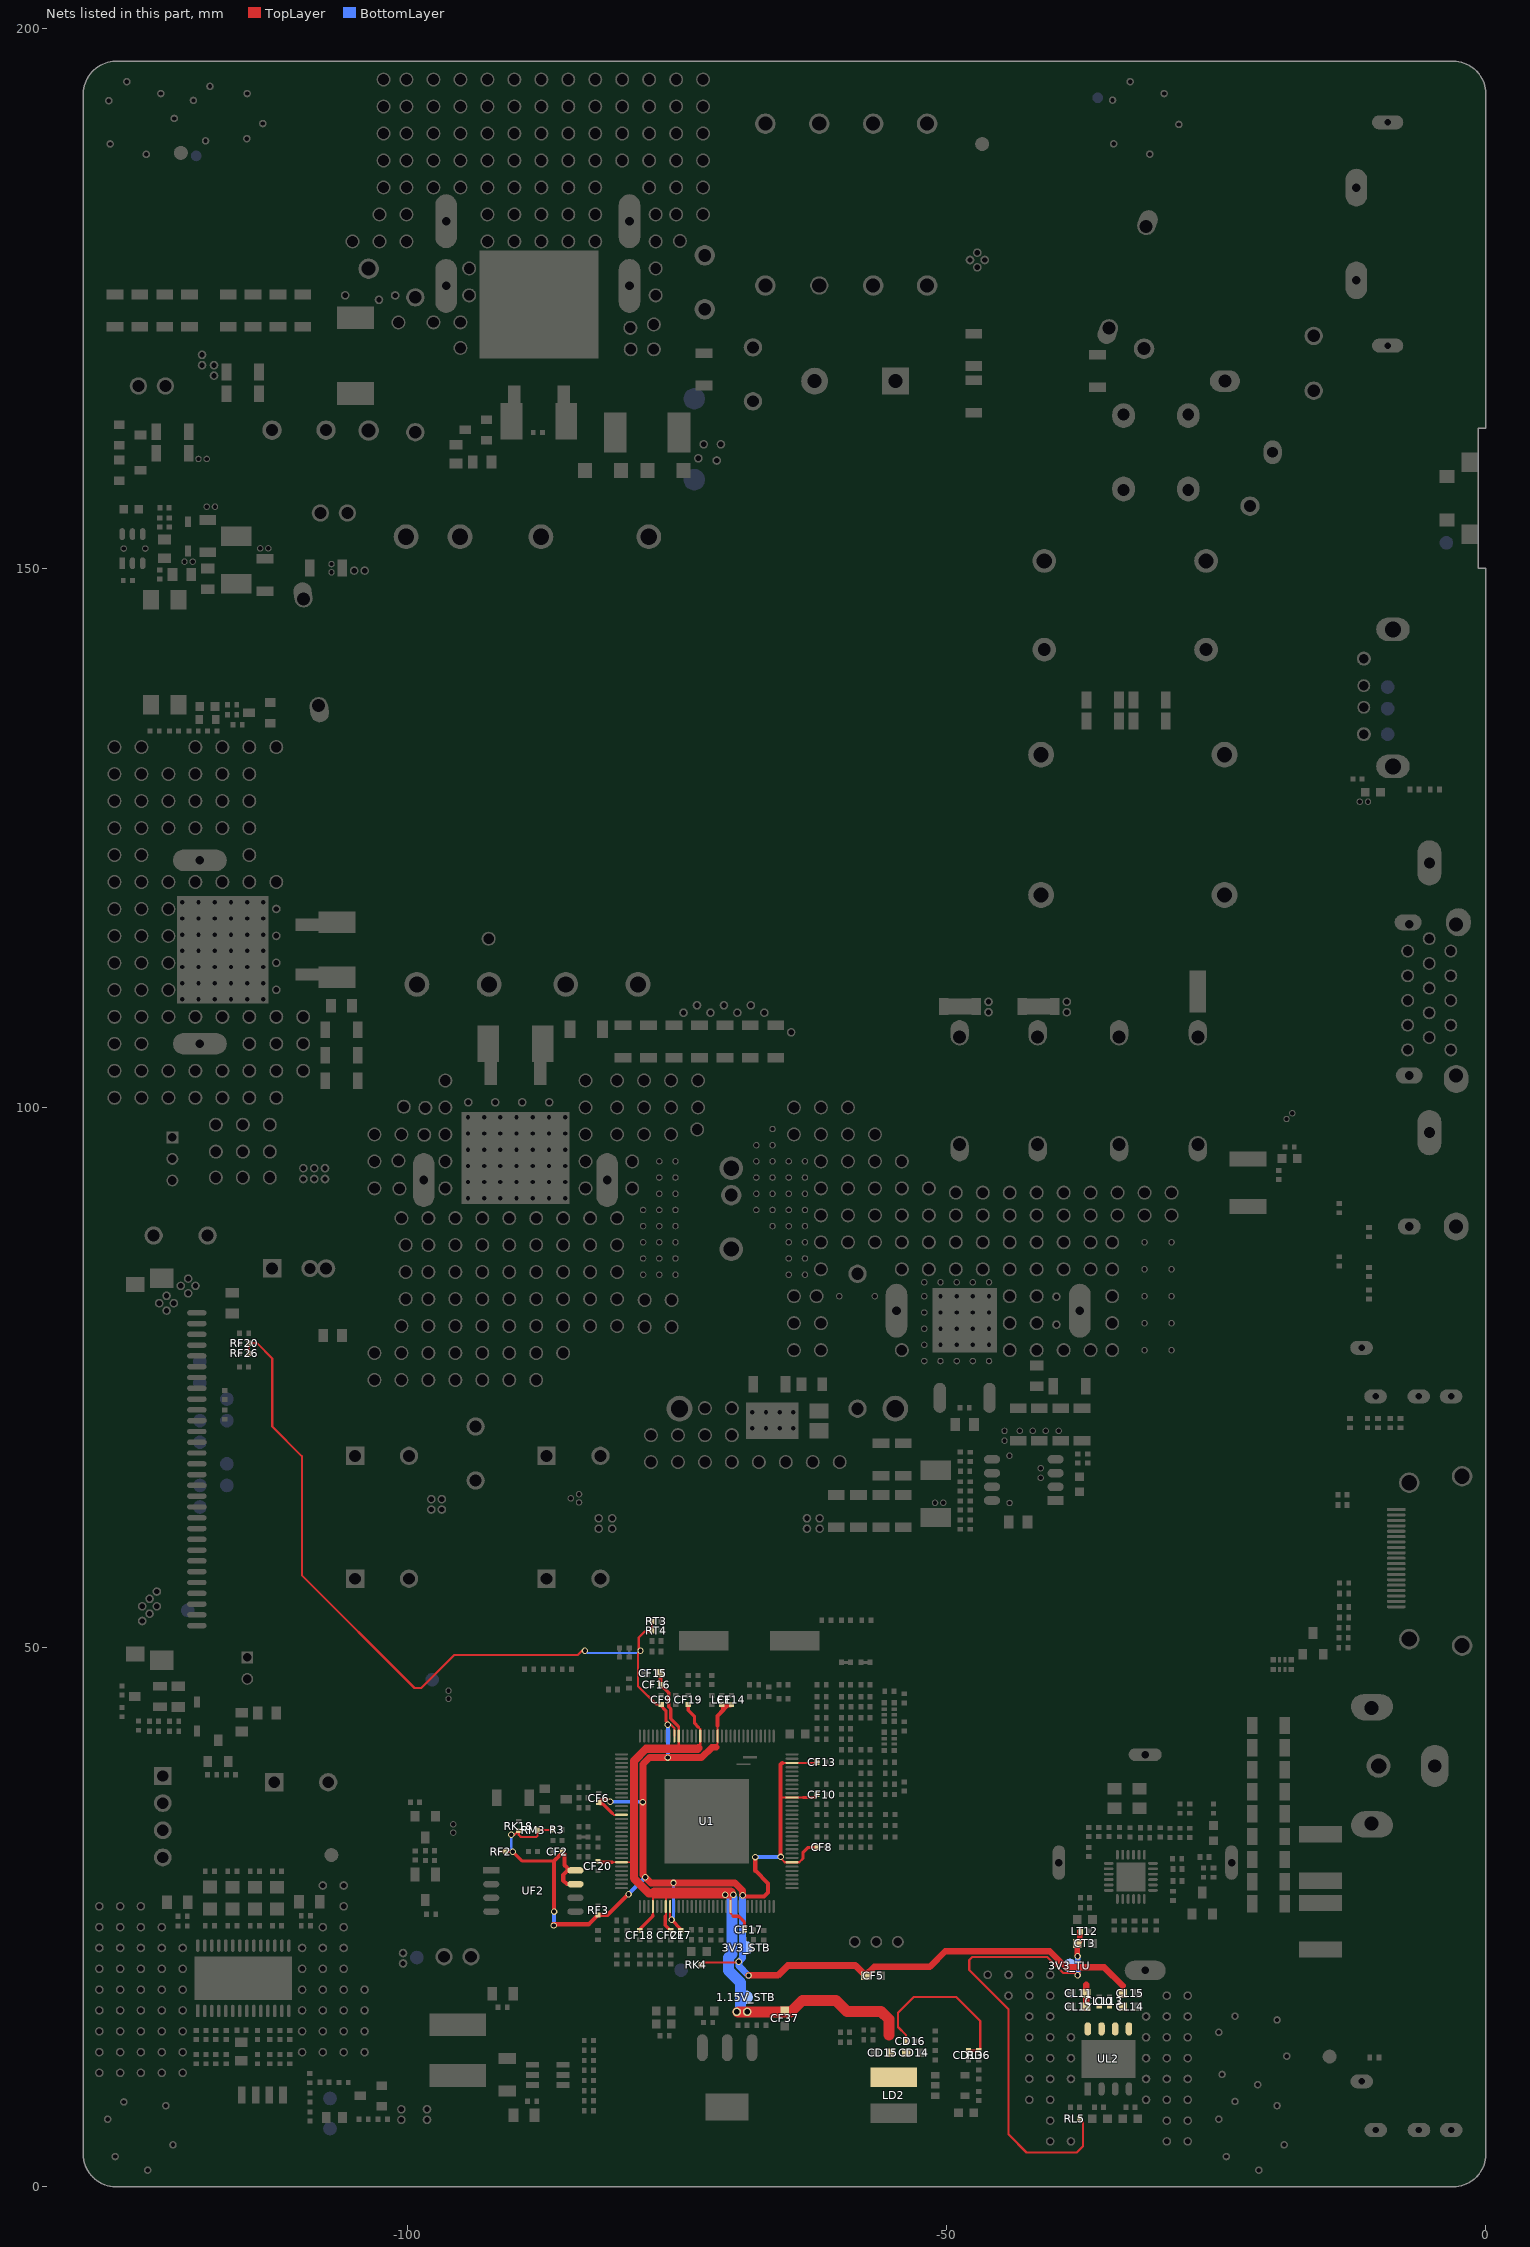
[diagram p0: the nets of this part, all layers, seen from the top]
# Altium PCB MISC84438.PcbDoc (part 6 of 15)
Units mm, origin at the board's own origin, x right, y up, seen from the top; angles counter-clockwise.
Board outline 130 x 197 mm, 2 copper layers (TopLayer, BottomLayer), stack 1.571 mm thick; 574 components, 314 nets, 2636 pads, 811 vias.

## Free pads (board coordinates)
  oval 5x4 on Keep-Out: 0(-15.5,5)
  round 4 on Keep-Out: 0(-3.5,192)
  round 1.2 on Top Solder: 1(-122.225,192.725)
  round 0.8 hole 0.5 paste-0.4 mask-0.4: VIA5(-128.524,10.541) VIA5(-128.524,12.471) VIA5(-128.524,14.402) VIA5(-128.524,16.332) VIA5(-128.524,18.263) VIA5(-128.524,20.193) VIA5(-128.524,22.123) VIA5(-128.524,24.054) VIA5(-128.524,25.984) VIA5(-126.594,10.541) VIA5(-126.594,12.471) VIA5(-126.594,14.402) VIA5(-126.594,16.332) VIA5(-126.594,18.263) VIA5(-126.594,20.193) VIA5(-126.594,22.123) VIA5(-126.594,24.054) VIA5(-126.594,25.984) VIA5(-124.663,10.541) VIA5(-124.663,12.471) VIA5(-124.663,14.402) VIA5(-124.663,16.332) VIA5(-124.663,18.263) VIA5(-124.663,20.193) VIA5(-124.663,22.123) VIA5(-124.663,24.054) VIA5(-124.663,25.984) VIA5(-124.547,52.432) VIA5(-124.547,53.797) VIA5(-123.865,53.115) VIA5(-123.865,54.48) VIA5(-123.182,53.797) VIA5(-123.182,55.162) VIA5(-122.972,81.89) VIA5(-122.733,10.541) VIA5(-122.733,12.471) VIA5(-122.733,14.402) VIA5(-122.733,16.332) VIA5(-122.733,18.263) VIA5(-122.733,20.193) VIA5(-122.733,22.123) VIA5(-122.733,24.054) VIA5(-122.29,81.207) VIA5(-122.29,82.572) VIA5(-121.607,81.89) VIA5(-120.972,83.49) VIA5(-120.802,10.541) VIA5(-120.802,12.471) VIA5(-120.802,14.402) VIA5(-120.802,16.332) VIA5(-120.802,18.263) VIA5(-120.802,20.193) VIA5(-120.802,22.123) VIA5(-120.29,84.172) VIA5(-120.29,82.807) VIA5(-119.607,83.49) VIA5(-118.999,168.834) VIA5(-118.999,169.799) VIA5(-117.892,167.875) VIA5(-117.892,168.84) VIA5(-109.728,12.471) VIA5(-109.728,14.402) VIA5(-109.728,16.332) VIA5(-109.728,18.263) VIA5(-109.728,20.193) VIA5(-109.728,22.123) VIA5(-107.798,12.471) VIA5(-107.798,14.402) VIA5(-107.798,16.332) VIA5(-107.798,18.263) VIA5(-107.798,20.193) VIA5(-107.798,22.123) VIA5(-107.798,24.054) VIA5(-107.798,27.915) VIA5(-105.867,12.471) VIA5(-105.867,14.402) VIA5(-105.867,16.332) VIA5(-105.867,18.263) VIA5(-105.867,20.193) VIA5(-105.867,22.123) VIA5(-105.867,24.054) VIA5(-105.867,25.984) VIA5(-105.867,27.915) VIA5(-104.897,149.801) VIA5(-103.937,12.471) VIA5(-103.937,14.402) VIA5(-103.937,16.332) VIA5(-103.937,18.263) VIA5(-103.932,149.801) VIA5(-100.517,6.198) VIA5(-100.517,7.163) VIA5(-100.368,20.688) VIA5(-100.368,21.653) VIA5(-98.146,6.198) VIA5(-98.146,7.163) VIA5(-97.739,62.763) VIA5(-97.739,63.729) VIA5(-96.774,62.763) VIA5(-96.774,63.729) VIA5(-82.233,60.985) VIA5(-82.233,61.951) VIA5(-80.989,60.985) VIA5(-80.989,61.951) VIA5(-74.371,108.814) VIA5(-73.121,109.505) VIA5(-71.871,108.814) VIA5(-70.621,109.505) VIA5(-69.431,16.197) VIA5(-69.371,108.814) VIA5(-68.466,16.197) VIA5(-68.121,109.505) VIA5(-66.871,108.814) VIA5(-64.4,107) VIA5(-62.928,60.985) VIA5(-62.928,61.951) VIA5(-61.759,60.985) VIA5(-61.759,61.951) VIA5(-47.814,178.588) VIA5(-47.132,177.906) VIA5(-47.132,179.271) VIA5(-46.449,178.588) VIA5(-46.177,19.634) VIA5(-46.101,108.865) VIA5(-46.101,109.83) VIA5(-44.247,17.704) VIA5(-44.247,19.634) VIA5(-42.316,8.052) VIA5(-42.316,9.982) VIA5(-42.316,11.913) VIA5(-42.316,13.843) VIA5(-42.316,15.773) VIA5(-42.316,17.704) VIA5(-42.316,19.634) VIA5(-40.386,4.191) VIA5(-40.386,6.121) VIA5(-40.386,8.052) VIA5(-40.386,9.982) VIA5(-40.386,11.913) VIA5(-40.386,13.843) VIA5(-40.386,15.773) VIA5(-40.386,17.704) VIA5(-40.386,19.634) VIA5(-39.8,79.9) VIA5(-39.8,82.5) VIA5(-38.837,108.865) VIA5(-38.837,109.83) VIA5(-38.456,4.191) VIA5(-38.456,9.982) VIA5(-38.456,11.913) VIA5(-38.456,13.843) VIA5(-31.496,8.052) VIA5(-31.496,9.982) VIA5(-31.496,11.913) VIA5(-31.496,13.843) VIA5(-31.496,15.773) VIA5(-29.566,4.191) VIA5(-29.566,6.121) VIA5(-29.566,8.052) VIA5(-29.566,9.982) VIA5(-29.566,11.913) VIA5(-29.566,13.843) VIA5(-29.566,15.773) VIA5(-29.566,17.704) VIA5(-27.635,4.191) VIA5(-27.635,6.121) VIA5(-27.635,8.052) VIA5(-27.635,9.982) VIA5(-27.635,11.913) VIA5(-27.635,13.843) VIA5(-27.635,15.773) VIA5(-27.635,17.704)
  round 1.3 hole 1 paste-0.65 mask-0.051: VIA5(-127.119,100.932) VIA5(-127.119,103.432) VIA5(-127.119,105.932) VIA5(-127.119,108.432) VIA5(-127.119,110.932) VIA5(-127.119,113.432) VIA5(-127.119,115.932) VIA5(-127.119,118.432) VIA5(-127.119,120.932) VIA5(-127.119,123.432) VIA5(-127.119,125.932) VIA5(-127.119,128.432) VIA5(-127.119,130.932) VIA5(-127.119,133.432) VIA5(-124.619,100.932) VIA5(-124.619,108.432) VIA5(-124.619,110.932) VIA5(-124.619,113.432) VIA5(-124.619,115.932) VIA5(-124.619,118.432) VIA5(-124.619,120.932) VIA5(-124.619,123.432) VIA5(-124.619,128.432) VIA5(-124.619,130.932) VIA5(-124.619,133.432) VIA5(-124.619,103.432) VIA5(-124.619,105.932) VIA5(-124.619,125.932) VIA5(-122.119,103.432) VIA5(-122.119,125.932) VIA5(-122.119,100.932) VIA5(-122.119,108.432) VIA5(-122.119,110.932) VIA5(-122.119,113.432) VIA5(-122.119,115.932) VIA5(-122.119,118.432) VIA5(-122.119,120.932) VIA5(-122.119,128.432) VIA5(-122.119,130.932) VIA5(-119.619,100.932) VIA5(-119.619,103.432) VIA5(-119.619,108.432) VIA5(-119.619,120.932) VIA5(-119.619,125.932) VIA5(-119.619,128.432) VIA5(-119.619,130.932) VIA5(-119.619,133.432) VIA5(-117.719,93.532) VIA5(-117.719,95.932) VIA5(-117.719,98.432) VIA5(-117.119,100.932) VIA5(-117.119,103.432) VIA5(-117.119,108.432) VIA5(-117.119,120.932) VIA5(-117.119,125.932) VIA5(-117.119,128.432) VIA5(-117.119,133.432) VIA5(-117.119,130.932) VIA5(-115.219,93.532) VIA5(-115.219,95.932) VIA5(-115.219,98.432) VIA5(-114.619,100.932) VIA5(-114.619,103.432) VIA5(-114.619,105.932) VIA5(-114.619,108.432) VIA5(-114.619,120.932) VIA5(-114.619,123.432) VIA5(-114.619,125.932) VIA5(-114.619,128.432) VIA5(-114.619,130.932) VIA5(-114.619,133.432) VIA5(-112.719,93.532) VIA5(-112.719,95.932) VIA5(-112.719,98.432) VIA5(-112.119,100.932) VIA5(-112.119,103.432) VIA5(-112.119,105.932) VIA5(-112.119,108.432) VIA5(-112.119,120.932) VIA5(-112.119,133.432) VIA5(-109.619,103.432) VIA5(-109.619,105.932) VIA5(-109.619,108.432) VIA5(-105.051,180.312) VIA5(-103.023,74.771) VIA5(-103.023,77.271) VIA5(-103.023,92.536) VIA5(-103.023,95.036) VIA5(-103.023,97.536) VIA5(-102.551,180.312) VIA5(-102.551,182.812) VIA5(-102.17,185.312) VIA5(-102.17,187.812) VIA5(-102.17,190.312) VIA5(-102.17,192.812) VIA5(-102.17,195.312) VIA5(-100.8,95.1) VIA5(-100.8,172.8) VIA5(-100.7,92.5) VIA5(-100.523,97.536) VIA5(-100.523,74.771) VIA5(-100.523,77.271) VIA5(-100.523,79.771) VIA5(-100.523,89.771) VIA5(-100.3,100.1) VIA5(-100.123,82.271) VIA5(-100.123,84.771) VIA5(-100.123,87.271) VIA5(-100.051,180.312) VIA5(-100.051,182.812) VIA5(-100.051,185.312) VIA5(-100.051,187.812) VIA5(-100.051,190.312) VIA5(-100.051,192.812) VIA5(-100.051,195.312) VIA5(-98.4,97.5) VIA5(-98.3,100) VIA5(-98.023,74.771) VIA5(-98.023,77.271) VIA5(-98.023,79.771) VIA5(-98.023,82.271) VIA5(-98.023,84.771) VIA5(-98.023,87.271) VIA5(-98.023,89.771) VIA5(-97.551,172.812) VIA5(-97.551,185.312) VIA5(-97.551,187.812) VIA5(-97.551,190.312) VIA5(-97.551,192.812) VIA5(-97.551,195.312) VIA5(-96.447,92.536) VIA5(-96.447,95.036) VIA5(-96.447,97.527) VIA5(-96.447,100.027) VIA5(-96.447,102.527) VIA5(-95.523,74.771) VIA5(-95.523,77.271) VIA5(-95.523,79.771) VIA5(-95.523,82.271) VIA5(-95.523,84.771) VIA5(-95.523,87.271) VIA5(-95.523,89.771) VIA5(-95.051,170.439) VIA5(-95.051,172.812) VIA5(-95.051,185.312) VIA5(-95.051,187.812) VIA5(-95.051,190.312) VIA5(-95.051,192.812) VIA5(-95.051,195.312) VIA5(-94.238,175.312) VIA5(-94.238,177.812) VIA5(-93.023,74.771) VIA5(-93.023,77.271) VIA5(-93.023,79.771) VIA5(-93.023,82.271) VIA5(-93.023,84.771) VIA5(-93.023,87.271) VIA5(-93.023,89.771) VIA5(-92.551,180.312) VIA5(-92.551,182.812) VIA5(-92.551,185.312) VIA5(-92.551,187.812) VIA5(-92.551,190.312) VIA5(-92.551,192.812) VIA5(-92.551,195.312) VIA5(-92.431,115.672) VIA5(-90.523,74.771) VIA5(-90.523,77.271) VIA5(-90.523,79.771) VIA5(-90.523,82.271) VIA5(-90.523,84.771) VIA5(-90.523,87.271) VIA5(-90.523,89.771) VIA5(-90.051,180.312) VIA5(-90.051,182.812) VIA5(-90.051,185.312) VIA5(-90.051,187.812) VIA5(-90.051,190.312) VIA5(-90.051,192.812) VIA5(-90.051,195.312) VIA5(-88.023,74.771) VIA5(-88.023,77.271) VIA5(-88.023,79.771) VIA5(-88.023,82.271) VIA5(-88.023,84.771) VIA5(-88.023,87.271) VIA5(-88.023,89.771) VIA5(-87.551,180.312) VIA5(-87.551,182.812) VIA5(-87.551,185.312) VIA5(-87.551,187.812) VIA5(-87.551,190.312) VIA5(-87.551,192.812) VIA5(-87.551,195.312) VIA5(-85.523,77.271) VIA5(-85.523,79.771) VIA5(-85.523,82.271) VIA5(-85.523,84.771) VIA5(-85.523,87.271) VIA5(-85.523,89.771) VIA5(-85.051,180.312) VIA5(-85.051,182.812) VIA5(-85.051,185.312) VIA5(-85.051,187.812) VIA5(-85.051,190.312) VIA5(-85.051,192.812) VIA5(-85.051,195.312) VIA5(-83.448,92.536) VIA5(-83.448,95.036) VIA5(-83.448,97.536) VIA5(-83.448,100.036) VIA5(-83.448,102.536) VIA5(-83.023,79.771) VIA5(-83.023,82.271) VIA5(-83.023,84.771) VIA5(-83.023,87.271) VIA5(-83.023,89.771) VIA5(-82.551,180.312) VIA5(-82.551,182.812) VIA5(-82.551,185.312) VIA5(-82.551,187.812) VIA5(-82.551,190.312) VIA5(-82.551,192.812) VIA5(-82.551,195.312) VIA5(-80.523,97.536) VIA5(-80.523,100.036) VIA5(-80.523,102.536) VIA5(-80.523,79.771) VIA5(-80.523,82.271) VIA5(-80.523,84.771) VIA5(-80.523,87.271) VIA5(-80.523,89.771) VIA5(-80.051,187.812) VIA5(-80.051,190.312) VIA5(-80.051,192.812) VIA5(-80.051,195.312) VIA5(-79.3,172.3) VIA5(-79.264,170.312) VIA5(-79.123,92.536) VIA5(-79.123,95.036) VIA5(-78.023,97.536) VIA5(-78.023,100.036) VIA5(-78.023,102.536) VIA5(-77.967,79.68) VIA5(-77.967,82.18) VIA5(-77.551,185.312) VIA5(-77.551,187.812) VIA5(-77.551,190.312) VIA5(-77.551,192.812) VIA5(-77.551,195.312) VIA5(-77.39,67.158) VIA5(-77.39,69.658) VIA5(-77.119,170.312) VIA5(-77.119,172.612) VIA5(-76.951,175.312) VIA5(-76.951,177.812) VIA5(-76.951,180.312) VIA5(-76.951,182.812) VIA5(-75.523,97.536) VIA5(-75.523,100.036) VIA5(-75.523,102.536) VIA5(-75.467,79.68) VIA5(-75.467,82.18) VIA5(-75.051,182.812) VIA5(-75.051,185.312) VIA5(-75.051,187.812) VIA5(-75.051,190.312) VIA5(-75.051,192.812) VIA5(-75.051,195.312) VIA5(-74.89,67.158) VIA5(-74.89,69.658) VIA5(-74.7,180.35) VIA5(-73.1,98) VIA5(-73.023,100.036) VIA5(-73.023,102.536) VIA5(-72.551,182.812) VIA5(-72.551,185.312) VIA5(-72.551,187.812) VIA5(-72.551,190.312) VIA5(-72.551,192.812) VIA5(-72.551,195.312) VIA5(-72.39,67.158) VIA5(-72.39,69.658) VIA5(-72.39,72.158) VIA5(-69.89,67.158) VIA5(-69.89,69.658) VIA5(-69.89,72.158) VIA5(-67.39,67.158) VIA5(-64.89,67.158) VIA5(-64.132,82.536) VIA5(-64.132,77.536) VIA5(-64.132,80.036) VIA5(-64.132,97.536) VIA5(-64.132,100.036) VIA5(-62.39,67.158) VIA5(-62.032,82.536) VIA5(-61.632,77.536) VIA5(-61.632,80.036) VIA5(-61.632,85.036) VIA5(-61.632,87.536) VIA5(-61.632,90.036) VIA5(-61.632,92.536) VIA5(-61.632,95.036) VIA5(-61.632,97.536) VIA5(-61.632,100.036) VIA5(-59.89,67.158) VIA5(-59.131,87.536) VIA5(-59.131,90.036) VIA5(-59.131,92.536) VIA5(-59.131,95.036) VIA5(-59.131,97.536) VIA5(-59.131,100.036) VIA5(-56.631,87.536) VIA5(-56.631,90.036) VIA5(-56.631,92.536) VIA5(-56.631,95.036) VIA5(-56.631,97.536) VIA5(-54.131,77.536) VIA5(-54.131,85.036) VIA5(-54.131,87.536) VIA5(-54.131,90.036) VIA5(-54.131,92.536) VIA5(-54.131,95.036) VIA5(-51.632,85.036) VIA5(-51.632,87.536) VIA5(-51.632,90.036) VIA5(-51.632,92.536) VIA5(-49.132,85.036) VIA5(-49.132,87.536) VIA5(-49.132,90.036) VIA5(-49.132,92.136) VIA5(-46.632,85.036) VIA5(-46.632,87.536) VIA5(-46.632,90.036) VIA5(-46.632,92.136) VIA5(-44.132,77.536) VIA5(-44.132,80.036) VIA5(-44.132,82.536) VIA5(-44.132,85.036) VIA5(-44.132,87.536) VIA5(-44.132,90.036) VIA5(-44.132,92.136) VIA5(-41.632,77.536) VIA5(-41.632,80.036) VIA5(-41.632,82.536) VIA5(-41.632,85.036) VIA5(-41.632,87.536) VIA5(-41.632,90.036) VIA5(-41.632,92.136) VIA5(-39.132,77.536) VIA5(-39.132,85.036) VIA5(-39.132,87.536) VIA5(-39.132,90.036) VIA5(-39.132,92.136) VIA5(-36.632,77.536) VIA5(-36.632,85.036) VIA5(-36.632,87.536) VIA5(-36.632,90.036) VIA5(-36.632,92.136) VIA5(-34.632,77.536) VIA5(-34.632,80.036) VIA5(-34.632,82.536) VIA5(-34.632,85.036) VIA5(-34.632,87.536) VIA5(-34.132,90.036) VIA5(-34.132,92.136) VIA5(-31.632,90.036) VIA5(-31.632,92.136) VIA5(-29.132,90.036) VIA5(-29.132,92.136)
  round 0.6 hole 0.4 paste-0.4 mask-0.4: VIA5(-126.263,151.841) VIA5(-124.257,151.841) VIA5(-120.821,116.05) VIA5(-120.821,111.55) VIA5(-120.821,113.05) VIA5(-120.821,114.55) VIA5(-120.821,117.55) VIA5(-120.821,110.05) VIA5(-120.821,119.05) VIA5(-120.625,150.628) VIA5(-119.863,150.628) VIA5(-119.329,160.147) VIA5(-119.321,110.05) VIA5(-119.321,111.55) VIA5(-119.321,113.05) VIA5(-119.321,114.55) VIA5(-119.321,116.05) VIA5(-119.321,117.55) VIA5(-119.321,119.05) VIA5(-118.567,155.723) VIA5(-118.567,160.147) VIA5(-117.821,116.05) VIA5(-117.821,110.05) VIA5(-117.821,111.55) VIA5(-117.821,113.05) VIA5(-117.821,114.55) VIA5(-117.821,117.55) VIA5(-117.821,119.05) VIA5(-117.805,155.723) VIA5(-116.321,110.05) VIA5(-116.321,111.55) VIA5(-116.321,113.05) VIA5(-116.321,114.55) VIA5(-116.321,116.05) VIA5(-116.321,117.55) VIA5(-116.321,119.05) VIA5(-114.821,110.05) VIA5(-114.821,113.05) VIA5(-114.821,114.55) VIA5(-114.821,117.55) VIA5(-114.821,111.55) VIA5(-114.821,116.05) VIA5(-114.821,119.05) VIA5(-113.614,151.854) VIA5(-113.321,110.05) VIA5(-113.321,111.55) VIA5(-113.321,113.05) VIA5(-113.321,114.55) VIA5(-113.321,116.05) VIA5(-113.321,117.55) VIA5(-113.321,119.05) VIA5(-112.852,151.854) VIA5(-107,149.638) VIA5(-107,150.4) VIA5(-96.152,45.212) VIA5(-96.152,45.974) VIA5(-95.72,32.817) VIA5(-95.72,33.579) VIA5(-94.343,93.115) VIA5(-94.343,96.115) VIA5(-94.343,91.615) VIA5(-94.343,94.615) VIA5(-94.343,97.615) VIA5(-94.343,99.115) VIA5(-92.843,93.115) VIA5(-92.843,96.115) VIA5(-92.843,91.615) VIA5(-92.843,94.615) VIA5(-92.843,97.615) VIA5(-92.843,99.115) VIA5(-91.343,91.615) VIA5(-91.343,93.115) VIA5(-91.343,94.615) VIA5(-91.343,96.115) VIA5(-91.343,97.615) VIA5(-91.343,99.115) VIA5(-89.843,91.615) VIA5(-89.843,93.115) VIA5(-89.843,94.615) VIA5(-89.843,96.115) VIA5(-89.843,97.615) VIA5(-89.843,99.115) VIA5(-88.343,91.615) VIA5(-88.343,93.115) VIA5(-88.343,94.615) VIA5(-88.343,96.115) VIA5(-88.343,97.615) VIA5(-88.343,99.115) VIA5(-86.843,91.615) VIA5(-86.843,94.615) VIA5(-86.843,93.115) VIA5(-86.843,96.115) VIA5(-86.843,97.615) VIA5(-86.843,99.115) VIA5(-85.343,91.615) VIA5(-85.343,93.115) VIA5(-85.343,94.615) VIA5(-85.343,96.115) VIA5(-85.343,97.615) VIA5(-85.343,99.115) VIA5(-84.811,63.805) VIA5(-84.049,63.424) VIA5(-84.049,64.186) VIA5(-78.115,84.535) VIA5(-78.115,86.035) VIA5(-78.115,87.535) VIA5(-78.115,89.035) VIA5(-78.115,90.535) VIA5(-76.615,84.535) VIA5(-76.615,86.035) VIA5(-76.615,87.535) VIA5(-76.615,89.035) VIA5(-76.615,90.535) VIA5(-76.615,92.035) VIA5(-76.615,93.535) VIA5(-76.615,95.035) VIA5(-75.115,84.535) VIA5(-75.115,86.035) VIA5(-75.115,87.535) VIA5(-75.115,89.035) VIA5(-75.115,90.535) VIA5(-75.115,92.035) VIA5(-75.115,93.535) VIA5(-75.115,95.035) VIA5(-70.51,27.048) VIA5(-69.748,27.048) VIA5(-68.001,70.284) VIA5(-68.001,71.784) VIA5(-67.615,90.535) VIA5(-67.615,92.035) VIA5(-67.615,93.535) VIA5(-67.615,95.035) VIA5(-67.615,96.535) VIA5(-66.73,70.284) VIA5(-66.73,71.784) VIA5(-66.115,89.035) VIA5(-66.115,90.535) VIA5(-66.115,92.035) VIA5(-66.115,93.535) VIA5(-66.115,95.035) VIA5(-66.115,96.535) VIA5(-66.115,98.035) VIA5(-65.459,71.784) VIA5(-65.459,70.284) VIA5(-64.615,84.535) VIA5(-64.615,86.035) VIA5(-64.615,87.535) VIA5(-64.615,89.035) VIA5(-64.615,90.535) VIA5(-64.615,92.035) VIA5(-64.615,93.535) VIA5(-64.615,95.035) VIA5(-64.187,70.284) VIA5(-64.187,71.784) VIA5(-63.115,84.535) VIA5(-63.115,86.035) VIA5(-63.115,87.535) VIA5(-63.115,89.035) VIA5(-63.115,90.535) VIA5(-63.115,92.035) VIA5(-63.115,93.535) VIA5(-63.115,95.035) VIA5(-52.05,76.525) VIA5(-52.05,78.025) VIA5(-52.05,79.525) VIA5(-52.05,81.025) VIA5(-52.05,82.525) VIA5(-52.05,83.825) VIA5(-51.054,63.386) VIA5(-50.55,76.525) VIA5(-50.55,78.025) VIA5(-50.55,79.525) VIA5(-50.55,81.025) VIA5(-50.55,82.525) VIA5(-50.55,83.825) VIA5(-50.292,63.386) VIA5(-49.05,76.525) VIA5(-49.05,78.025) VIA5(-49.05,79.525) VIA5(-49.05,81.025) VIA5(-49.05,82.525) VIA5(-49.05,83.825) VIA5(-47.55,76.525) VIA5(-47.55,78.025) VIA5(-47.55,79.525) VIA5(-47.55,81.025) VIA5(-47.55,82.525) VIA5(-47.55,83.825) VIA5(-46.05,76.525) VIA5(-46.05,78.025) VIA5(-46.05,83.825) VIA5(-46.05,79.525) VIA5(-46.05,81.025) VIA5(-46.05,82.525) VIA5(-44.615,69.151) VIA5(-44.615,70.053) VIA5(-44.158,67.754) VIA5(-44.146,63.372) VIA5(-43.199,70.053) VIA5(-41.999,70.053) VIA5(-41.262,65.697) VIA5(-41.262,66.599) VIA5(-40.799,70.053) VIA5(-39.599,70.053) VIA5(-31.632,77.536) VIA5(-31.632,80.036) VIA5(-31.632,82.536) VIA5(-31.632,85.036) VIA5(-31.632,87.536) VIA5(-29.132,77.536) VIA5(-29.132,80.036) VIA5(-29.132,82.536) VIA5(-29.132,85.036) VIA5(-29.132,87.536) VIA5(-18.475,98.964) VIA5(-17.936,99.502) VIA5(-11.684,128.372) VIA5(-10.922,128.372)
  round 0.8 hole 0.5 paste-0.65 mask-0.051: VIA5(-112.119,110.932) VIA5(-112.119,113.432) VIA5(-112.119,115.932) VIA5(-112.119,118.432) VIA5(-109.6,93.4) VIA5(-109.6,94.4) VIA5(-108.6,93.4) VIA5(-108.6,94.4) VIA5(-107.6,93.4) VIA5(-107.6,94.4) VIA5(-105.737,175.312) VIA5(-102.6,174.9) VIA5(-101.1,175.3) VIA5(-94.323,100.508) VIA5(-91.823,100.508) VIA5(-89.323,100.508) VIA5(-86.823,100.508) VIA5(-73,160.2) VIA5(-72.5,161.5) VIA5(-71.3,160) VIA5(-70.9,161.5)
  round 0.6 hole 0.4 paste-0.65 mask-0.051: VIA5(-59.931,82.536) VIA5(-56.631,82.536)

## Via types
v1: diameter 0.6, hole 0.4, TopLayer to BottomLayer, tented both sides, 780 vias
v2: diameter 0.7, hole 0.5, TopLayer to BottomLayer, tented both sides, 15 vias
v3: diameter 0.8, hole 0.6, TopLayer to BottomLayer, tented both sides, 12 vias
v4: diameter 0.8, hole 0.5, TopLayer to BottomLayer, tented both sides, 4 vias

## Nets (pads, with @x,y where several pads share a name; then routed paths per layer and width w, separated by ;. In a path a pad name is that pad's centre, name@x,y a point inside that pad or via, vN(x,y) a via of type N, cw(c..) or ccw(c..) an arc to the next point about the centre after c; other vN are vias at no path point)
1.15V_STB: 1.15V_STB.1 CD13.1 CD14.2 CD15.2 CD16.2 CF15.1 CF16.2 CF17.2 CF18.2 CF19.2 CF20.2 CF21.2 CF37.1 LD2.2 pad.VIA5@-68.466,16.197 pad.VIA5@-69.431,16.197 pad.VIA5@-69.748,27.048 pad.VIA5@-70.51,27.048 RD6.2 U1.50 U1.55 U1.90 U1.100 U1.103 U1.118 | length 96.4
  TopLayer w0.178: -80.95,30.071 U1.90@-80.112,30.071 -79.324,30.071 ; -77.212,25.143 U1.100@-77.212,25.971 -77.212,26.769 ; -76.012,25.067 U1.103@-76.012,25.971 -76.012,26.769 ; pad.VIA5@-70.012,27.055 U1.118@-70.012,25.971 -70.012,25.331 -69.748,25.067
  TopLayer w0.203: -74.901,42.726 -74.812,42.637 U1.55@-74.812,41.771 -74.812,40.589 -74.812,40.324 ; -73.007,42.602 -72.812,42.408 U1.50@-72.812,41.771 -72.812,40.826 ; CD16.2@-53.765,13.487 CD16.2@-53.765,13.634 ; CD16.2@-53.734,13.538 -53.734,14.046 -54.483,14.795 -54.483,16.112 -53.024,17.57 -49.088,17.57 -46.867,15.349 -46.867,12.753 RD6.2@-47.015,12.604 CD13.1@-47.955,12.604
  TopLayer w0.305: CF20.2@-82.296,30.071 -80.95,30.071 ; CF18.2@-78.34,23.739 -78.34,23.943 -77.212,25.071 -77.212,25.143 ; CF15.1@-76.51,47.574 CF15.1@-76.461,47.525 ; CF16.2@-76.486,46.507 -75.751,45.771 -75.751,44.468 -75.565,44.282 -75.565,43.389 -74.901,42.726 ; -76.055,25.092 -76.055,24.23 CF21.2@-75.552,23.727 ; CF19.2@-73.939,44.685 -73.939,44.155 -73.343,43.558 -73.343,42.938 -73.007,42.603 ; -69.748,25.067 -69.253,25.067 -68.726,24.54 CF17.2@-68.726,23.975
  TopLayer w0.381: CF15.1@-76.51,47.574 -76.51,46.53 CF16.2@-76.486,46.507
  TopLayer w0.762: -77.064,27.206 -77.598,27.206 -78.969,28.576 -78.969,39.471 -77.851,40.589 -74.812,40.589 -73.047,40.589 -72.973,40.663
  TopLayer w1.016: -77.064,27.206 -70.028,27.206 ; pad.VIA5@-69.317,16.197 pad.VIA5@-68.466,16.197 -64.432,16.197 -63.36,17.269 -60.23,17.269 -59.198,16.237 -56.054,16.237 -55.334,15.517 -55.334,14.072
  BottomLayer w1.016: -69.876,26.768 -69.876,21.552 -70.193,21.235 -70.193,20.048 -69.075,18.93 pad.VIA5@-69.075,16.332
3V3_STB: 3V3_STB.1 CF2.2 CF5.1 CF6.2 CF7.2 CF8.2 CF9.2 CF10.2 CF13.2 CF14.2 CL13.1 CL14.1 CL15.2 LF1.1 R3.2 RF2.2 RF2.3 RF3.2 RF20.2 RF26.1 RK4.2 RK18.2 RM3.1 RT3.1 RT4.1 U1.7 U1.22 U1.30 U1.46 U1.56 U1.79 U1.104 UF2.7 UF2.8 UL2.5 UL2.6 | length 235.7
  TopLayer w0.152: U1.46@-71.212,41.771 U1.46@-71.198,41.784
  TopLayer w0.178: -80.959,34.598 -80.828,34.468 -80.115,34.468 U1.79@-80.112,34.471
  TopLayer w0.191: v1@-75.612,24.873 U1.104@-75.612,25.971 ; -71.374,40.881 -71.212,41.043 U1.46@-71.212,41.771
  TopLayer w0.198: -65.216,39.271 U1.30@-64.312,39.271 -61.995,39.271 CF13.2@-61.886,39.271
  TopLayer w0.203: RF26.1@-114.641,77.203 RF26.1@-114.668,77.229 RF20.2@-114.668,78.169 -113.895,78.169 -112.485,76.759 -112.485,70.453 -109.747,67.715 -109.747,56.673 -99.302,46.228 -98.669,46.228 -95.621,49.276 -84.175,49.276 -83.794,49.657 -83.502,49.657 v1@-83.477,49.657 ; v1(-90.339,32.609) -90.029,32.609 RK18.2@-89.637,33.001 -89.637,32.614 -89.433,32.41 -88.011,32.41 -87.891,32.531 RM3.1@-87.891,33.045 ; v1@-90.22,31.064 v1(-90.195,31.039) ; RM3.1@-87.891,33.071 R3.2@-86.48,33.071 ; v1@-78.383,49.67 -78.519,49.806 -78.519,50.904 -77.959,51.464 -77.304,51.464 RT4.1@-77.304,51.515 RT3.1@-77.304,52.417 ; v1(-78.358,49.67) -78.582,49.446 -78.582,46.385 -76.881,44.685 CF9.2@-76.579,44.685 ; v1@-75.538,42.824 -75.212,42.498 U1.56@-75.212,41.771 ; RK4.2@-72.778,20.559 -72.568,20.768 v1@-69.24,20.768 ; U1.46@-71.212,41.771 -71.212,42.721 -71.173,42.761 ; v1@-65.365,30.441 -64.995,30.071 U1.7@-64.312,30.071 -63.642,30.071 -63.297,30.416 ; -65.227,36.071 U1.22@-64.312,36.071 -63.273,36.071
  TopLayer w0.305: RF2.2@-90.875,31.064 v1@-90.22,31.064 ; v1(-90.195,31.039) -89.344,30.188 -86.373,30.188 ; CF6.2@-82.22,35.592 -82.109,35.481 -81.841,35.481 -80.959,34.598 ; CF6.2@-82.194,35.649 -81.978,35.865 v1@-81.364,35.865 ; CF9.2@-76.579,44.685 -76.504,44.61 -75.997,44.103 -75.997,43.18 v1@-75.819,43.002 ; v1(-75.476,24.737) -74.612,23.873 CF7.2@-74.612,23.727 ; -63.297,30.416 -63.297,30.962 -62.814,31.445 CF8.2@-61.995,31.445 ; -63.273,36.071 -62.246,36.071 CF10.2@-61.995,36.322
  TopLayer w0.381: v1@-86.462,24.325 -86.385,24.325 -83.149,24.325 RF3.2@-82.296,25.178 -81.422,25.178 v1@-79.486,27.114 ; v1(-86.373,25.502) -86.373,30.188 -85.63,30.93 CF2.2@-85.63,31.064 -85.407,30.841 -85.407,29.794 UF2.8@-84.925,29.312 ; UF2.7@-84.39,28.042 -85.179,28.042 -85.522,28.384 -85.522,28.892 -85.103,29.312 UF2.8@-84.925,29.312 ; UF2.8@-84.39,29.312 UF2.8@-84.925,29.312 ; -71.231,42.752 -71.231,43.627 -70.688,44.171 ; v1@-68.754,26.888 -66.911,26.888 -66.521,27.278 -66.521,28.09 -67.716,29.285 v1(-67.716,30.553) ; v1@-65.371,30.564 -65.371,39.116 -65.216,39.271 ; -70.688,44.171 -70.507,44.352 -70.276,44.583 ; -70.688,44.171 -70.688,44.43 -70.841,44.583 -70.276,44.583 ; -70.276,44.583 CF14.2@-70.073,44.583 ; CF14.2@-70.073,44.583 -69.97,44.685 CF14.2@-69.926,44.685 -70.029,44.583 CF14.2@-70.073,44.583
  TopLayer w0.61: v1@-68.343,19.576 -65.616,19.576 -64.697,20.495 -58.438,20.495 CF5.1@-57.501,19.558 -56.669,20.39 -51.533,20.39 -50.104,21.819 -40.419,21.819 -38.945,20.345 -35.395,20.345 -33.663,18.613
  TopLayer w0.635: -78.118,28.893 -78.118,35.649 -78.118,39.154 -77.509,39.763 -75.819,39.763 -72.705,39.763 -71.742,40.726 -71.361,40.726 ; v1@-77.902,28.677 -77.383,28.158 -75.298,28.158 -69.582,28.158 -68.889,27.465 v1(-68.889,27.023)
  BottomLayer w0.203: v1(-90.339,32.609) -90.339,31.182 v1(-90.195,31.039) ; v1(-83.502,49.682) -83.292,49.472 v1@-78.582,49.472
  BottomLayer w0.305: v1(-81.165,35.666) v1@-78.173,35.666 ; v1@-75.527,24.788 -75.298,25.016 v1(-75.298,28.153)
  BottomLayer w0.381: v1(-86.385,24.206) -86.373,24.219 v1(-86.373,25.502) ; v1(-79.464,27.114) v1(-77.902,28.677) ; v1(-75.819,39.776) v1(-75.819,42.824) ; v1@-67.706,30.564 v1(-65.365,30.564)
  BottomLayer w0.635: v1(-68.889,27.023) -68.889,22.123 -68.889,21.192 v1(-69.24,20.841) -69.24,20.442 v1@-68.369,19.571
  other v1: -68.343,19.571 -78.156,35.649
3V3_TU: 3V3_TU.1 CL10.2 CL11.1 CL12.1 CT3.1 LT12.1 RL5.2 UL2.7 UL2.8 | length 45.4
  TopLayer w0.203: RL5.2@-37.662,6.299 -37.338,5.975 -37.338,3.747 -37.922,3.162 -42.568,3.162 -44.234,4.828 -44.234,16.416 -47.892,20.074 -47.892,21.006 -47.612,21.285 -40.64,21.285 -39.166,19.812 -37.617,19.812
  TopLayer w0.508: v1(-37.846,21.361) -37.867,21.382 CT3.1@-37.867,22.543 -37.636,22.773 LT12.1@-37.636,23.66
  TopLayer w0.61: CL12.1@-37.038,16.688 CL11.1@-37.038,17.907 -37.038,18.704
  BottomLayer w0.508: v1(-37.846,19.609) v1(-37.846,21.361)